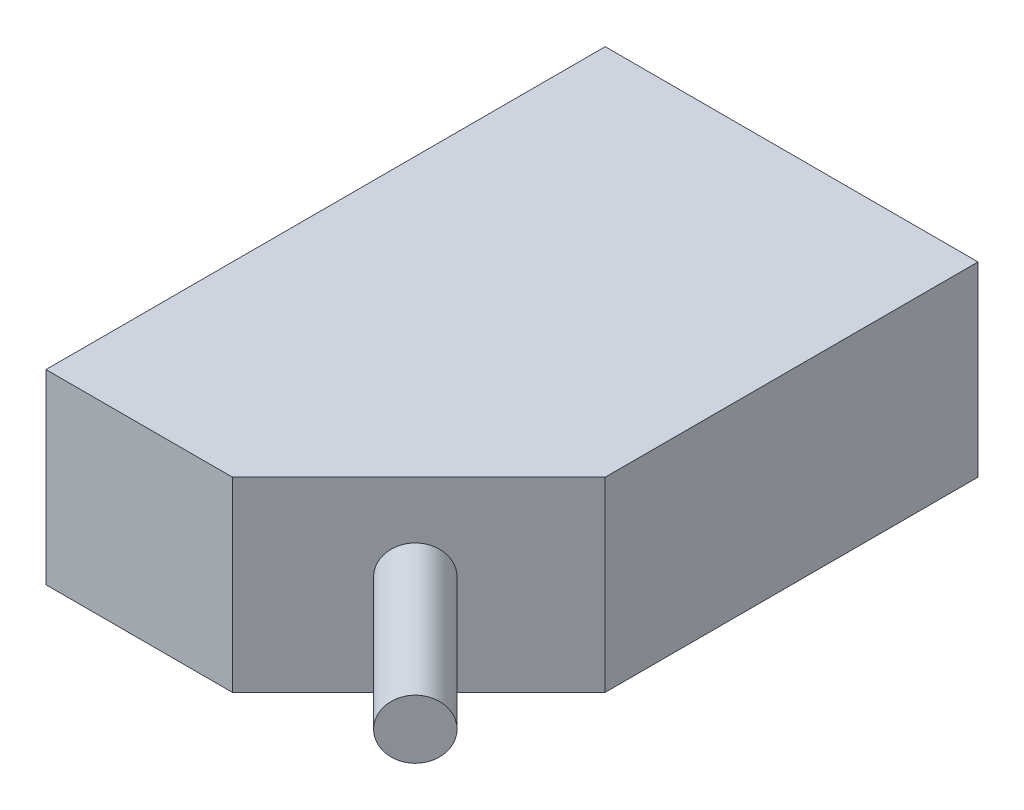
SolidWorks part; units mm, degrees
material "Q235-A"
ref_plane "Front Plane" through (0, 0, 0) normal (0, 0, 1) x (1, 0, 0)
ref_plane "Top Plane" through (0, 0, 0) normal (0, 1, 0) x (1, 0, 0)
ref_plane "Right Plane" through (0, 0, 0) normal (1, 0, 0) x (0, 0, -1)
sketch "Sketch1" plane through (0, 0, 0) normal (0, 1, 0) x (1, 0, 0)
  line L1 (0, 0) -> (20, 0)
  line L2 (0, 0) -> (0, -30)
  line L3 (0, -30) -> (20, -30)
  line L4 (20, 0) -> (20, -30)
  dimension "D1" = 20
  dimension "D2" = 30
extrude "Boss-Extrude1" add sketch "Sketch1" along normal blind 10
chamfer "Chamfer1" distance 10 angle 45 1 edges at (20, 5, 30)
sketch "Sketch2" plane through (20, 0, 20) normal (0.7071, 0, 0.7071) x (0.7071, 0, -0.7071)
  circle A0 centre (-7.2036, 5.3603) radius 1.5843
extrude "Boss-Extrude2" add sketch "Sketch2" along normal blind 10
